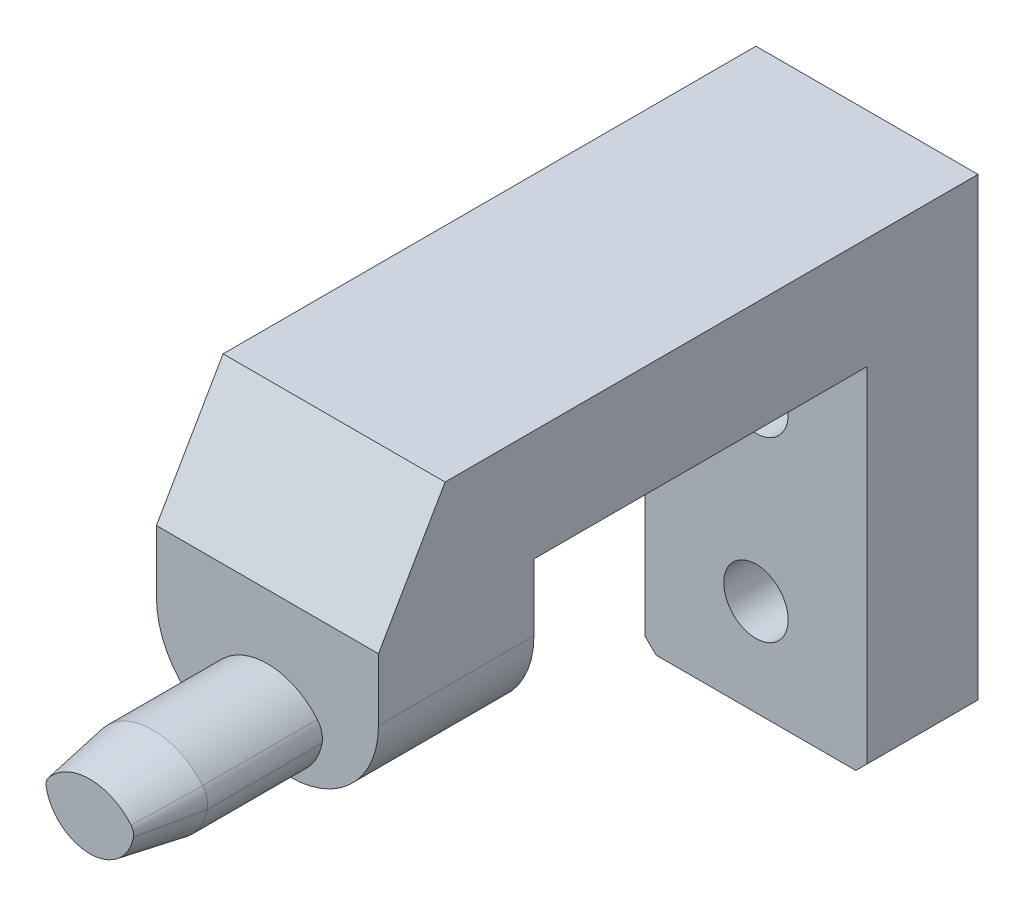
SolidWorks part; units mm, degrees
material "Cr12MoV"
ref_plane "Front Plane" through (0, 0, 0) normal (0, 0, 1) x (1, 0, 0)
ref_plane "Top Plane" through (0, 0, 0) normal (0, 1, 0) x (1, 0, 0)
ref_plane "Right Plane" through (0, 0, 0) normal (1, 0, 0) x (0, 0, -1)
sketch "Sketch1" plane through (0, 0, 0) normal (0, 1, 0) x (1, 0, 0)
  line L1 (-5, -10) -> (5, -10)
  line L2 (-5, -10) -> (-5, 10)
  line L3 (-5, 10) -> (5, 10)
  line L4 (5, -10) -> (5, 10)
  line L5 (-5, -10) -> (5, 10) construction
  line L6 (-5, 10) -> (5, -10) construction
  point P0 (0, 0)
  dimension "D1" = 10
  dimension "D2" = 20
extrude "Boss-Extrude1" add sketch "Sketch1" along normal blind 5
sketch "Sketch2" plane through (0, 0, 0) normal (0, -1, 0) x (-1, 0, 0)
  line L0 (5, 10) -> (5, -10) construction
  line L1 (-5, 10) -> (5, 10)
  line L2 (-5, 10) -> (-5, 5)
  line L3 (-5, 5) -> (5, 5)
  line L4 (5, 10) -> (5, 5)
  dimension "D1" = 5
extrude "Boss-Extrude2" add sketch "Sketch2" along normal blind 16
hole_wizard "M2.5 Clearance Hole1" positions "Sketch4" profile "Sketch3" hole size "M2.5" standard "Iso" end condition through all
sketch "Sketch4" plane through (0, 0, -5) normal (0, 0, 1) x (1, 0, 0)
  line L0 (5, -16) -> (-5, -16) construction
  point P0 (0, -11.65)
  point P5 (0, -3.65)
  dimension "D1" = 8
  dimension "D2" = 4.35
sketch "Sketch3" plane through (0, -11.65, -5) normal (1, 0, 0) x (0, -1, 0)
  line L0 (0, 0) -> (0, 5)
  line L1 (0, 5) -> (1.45, 5)
  line L2 (1.45, 5) -> (1.45, 0)
  line L5 (1.45, 0) -> (0, 0)
  line L11 (0, -6.35) -> (0, 107.95) construction
  dimension "通孔孔直径" = 2.9
  dimension "通孔孔深度" = 5
sketch "Sketch6" plane through (0, 0, 10) normal (0, 0, 1) x (1, 0, 0)
  line L0 (5, 5) -> (5, 0) construction
  line L1 (-5, 5) -> (5, 5)
  line L2 (-5, 5) -> (-5, -7)
  line L3 (-5, -7) -> (5, -7)
  line L4 (5, 5) -> (5, -7)
  dimension "D1" = 12
extrude "Boss-Extrude4" add sketch "Sketch6" along normal blind 7
chamfer "Chamfer1" distance 3 angle 60 1 edges at (0, 5, 17)
fillet "Fillet1" radius 4 2 edges at (5, -7, 13.5) (-5, -7, 13.5)
chamfer "Chamfer2" distance 0.5 angle 45 2 edges at (5, -16, -7.5) (-5, -16, -7.5)
sketch "Sketch8" plane through (0, 0, 17) normal (0, 0, 1) x (1, 0, 0)
  line L0 (0, 0) -> (0, -7) construction
  line L1 (-1, -7) -> (1, -7) construction
  arc A0 (-2.5, -4.5) -> (2.5, -4.5) centre (0, -4.5) ccw
  arc A1 (-2.5, -4.5) -> (2.5, -4.5) centre (0, -6) cw
  dimension "D1" = 5
  dimension "D3" = 1.5
  dimension "D2" = 2.5
extrude "Boss-Extrude6" add sketch "Sketch8" along normal blind 8
fillet "Fillet3" radius 1 2 edges at (-2.5, -4.5, 21) (2.5, -4.5, 21)
chamfer "Chamfer3" distance 0.5 angle 80 4 edges at (0, -3.0845, 25) (-2.4423, -4.5263, 25) (2.4423, -4.5263, 25) (0, -7, 25)
sketch "Sketch9" plane through (0, 0, -10) normal (0, 0, -1) x (-1, 0, 0)
  circle A0 centre (0, -3.65) radius 2
  circle A1 centre (0, -11.65) radius 2
  dimension "D1" = 4
extrude "Cut-Extrude1" cut sketch "Sketch9" against normal blind 2.1
